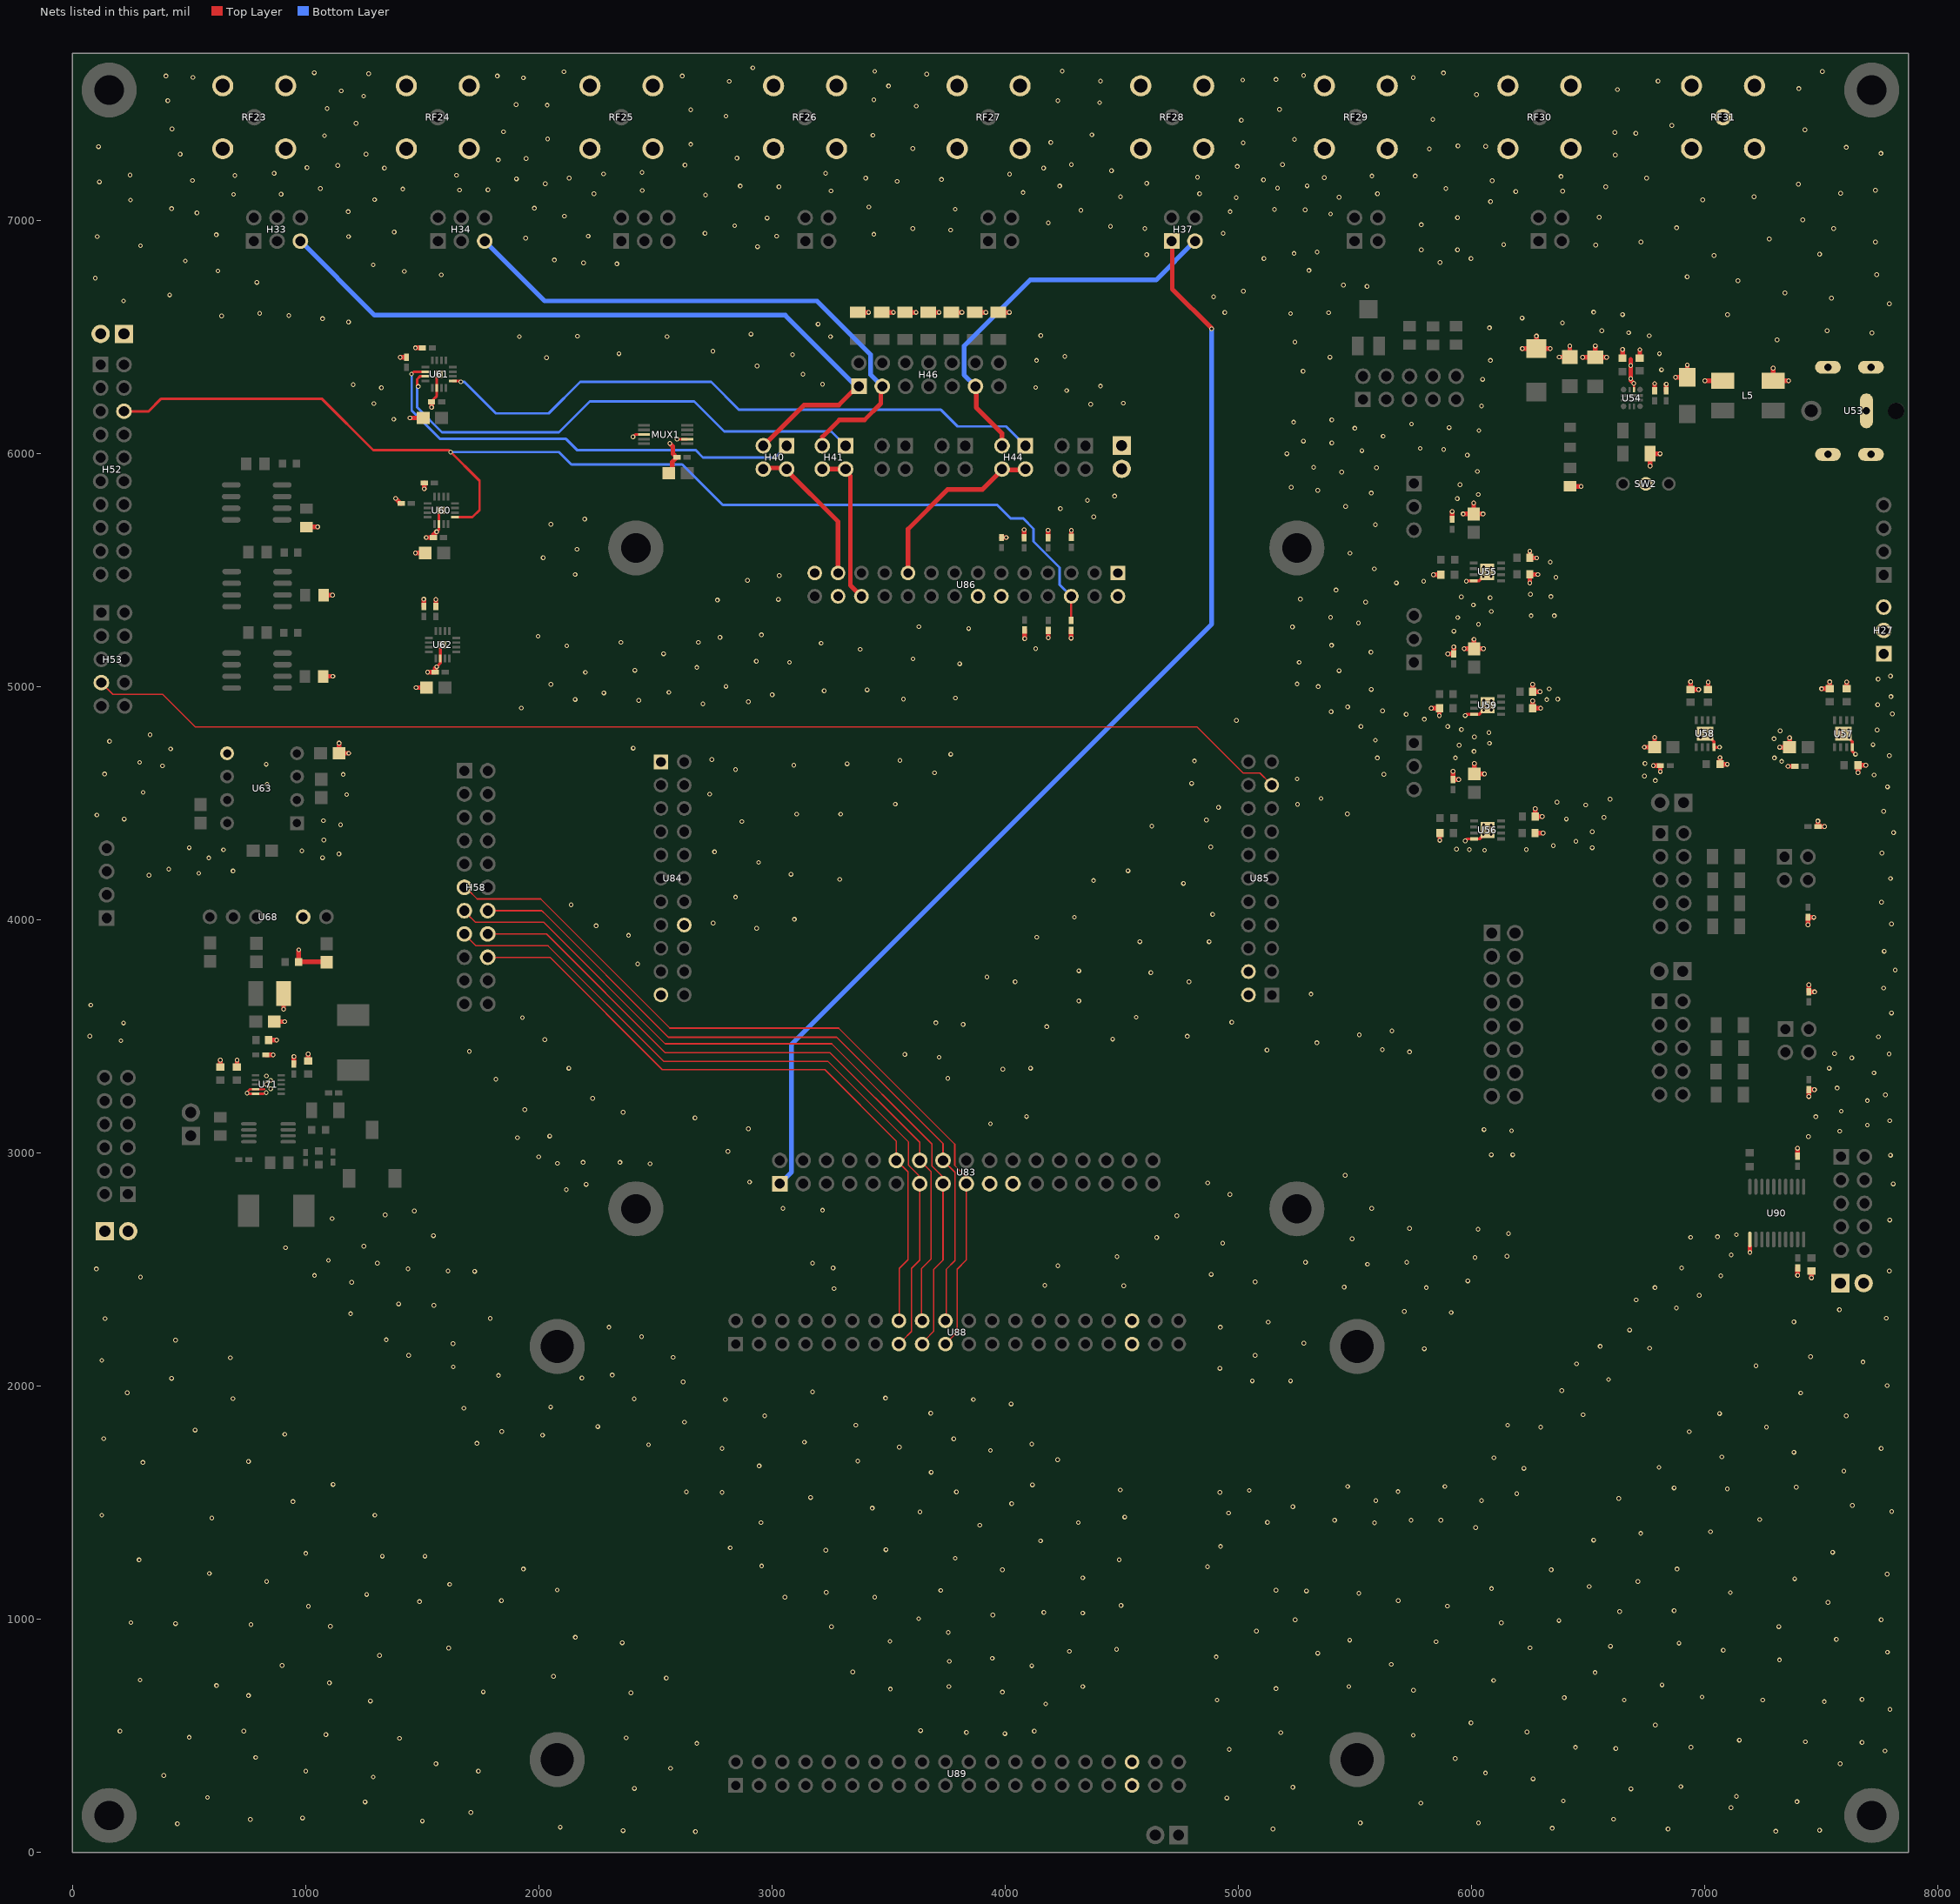
[diagram p0: the nets of this part, all layers, seen from the top]
# Altium PCB MISC62793.pcbdoc (part 5 of 6)
Units mil, origin at the board's own origin, x right, y up, seen from the top; angles counter-clockwise.
Board outline 7874.02 x 7716.54 mil, 4 copper layers (Top Layer, GND, VCC, Bottom Layer); 201 components, 197 nets, 941 pads, 1215 vias.

## Via types
v1: diameter 20, hole 12, Top Layer to Bottom Layer, 1215 vias

## Nets (pads, with @x,y where several pads share a name; then routed paths per layer and width w, separated by ;. In a path a pad name is that pad's centre, name@x,y a point inside that pad or via, vN(x,y) a via of type N, cw(c..) or ccw(c..) an arc to the next point about the centre after c; other vN are vias at no path point) (continued)
VSS: C126.1 C129.1 C130.1 C131.1 C132.1 C133.1 C134.1 C135.1 C136.1 C137.1 C138.1 C139.1 C140.1 C141.1 C142.1 C143.1 C144.1 C145.1 C146.1 C147.1 C148.1 C149.1 C150.1 C151.1 C152.1 C157.1 C158.1 C159.1 C163.1 C182.1 C183.1 C184.1 C185.2 C192.2 C193.2 C194.2 C195.1 C196.2 C197.1 C198.1 C199.1 C200.1 C201.1 C202.2 C203.2 C204.2 C205.2 C206.2 C207.2 C208.2 C215.1 C216.1 C217.1 C218.1 C219.1 C220.1 C221.1 C223.1 C224.1 C225.1 C226.1 C227.1 C228.1 D4.2 D5.1 H1.1 H1.2 H2.1 H2.2 H3.1 H3.2 H4.1 H4.2 H27.1 H27.2 H27.3 L5.2 L5.3 MUX1.3 MUX1.7 R91.1 R93.1 R96.1 R97.1 R98.1 R111.1 R113.1 R115.1 R120.2 R121.2 R122.2 R123.2 R124.2 R125.2 R126.2 R127.2 R134.2 R135.1 RF23.2 RF23.3 RF23.4 RF23.5 RF24.2 RF24.3 RF24.4 RF24.5 RF25.2 RF25.3 RF25.4 RF25.5 RF26.2 RF26.3 RF26.4 RF26.5 RF27.2 RF27.3 RF27.4 RF27.5 RF28.2 RF28.3 RF28.4 RF28.5 RF29.2 RF29.3 RF29.4 RF29.5 RF30.2 RF30.3 RF30.4 RF30.5 RF31.1 RF31.2 RF31.3 RF31.4 RF31.5 SW2.2 U53.2 U53.3 U54.8 U55.4 U55.9 U56.4 U56.9 U57.4 U57.9 U58.4 U58.9 U59.4 U59.9 U60.6 U60.17 U61.6 U61.17 U62.6 U62.17 U63.5 U68.2 U71.4 U71.5 U71.11 U82.2 U83.10 U83.11 U84.1 U84.16 U84.21 U85.2 U85.4 U86.1 U86.2 U86.12 U86.14 U86.26 U86.27 U88.35 U88.36 U89.35 U89.36 U90.11 | length 5722.7
  Top Layer w10: v1(749,3256) 749,3260 762.33,3273.33 U71.4@785.07,3273.33 821.67,3273.33 ; v1@750,3253.65 U71.5@785.07,3253.65 819.35,3253.65 ; v1(6696,6300.7) 6696.39,6300.31 U54.8@6696.39,6273.62
  Top Layer w11: C221.1@1544,6228 1562.85,6246.85 U61.6@1562.85,6281.39 U61.17@1562.85,6325.85 ; v1(1562,5664) 1572.28,5674.28 U60.6@1572.28,5697.2 U60.17@1572.28,5742.72 ; v1(2404,6071) 2414.06,6081.06 MUX1.3@2451.49,6081.06 ; v1(2593.37,6061.37) MUX1.7@2636.53,6061.37
  Top Layer w12: v1(1562.48,5085) 1577.9,5100.42 U62.6@1577.9,5119.95 U62.17@1577.9,5164.1
  Top Layer w13: v1(5973,4338) 5981.59,4346.59 U56.4@6010.83,4346.59 6034.59,4346.59 U56.9@6042,4354 ; v1(5973,4876) 5978.59,4881.59 U59.4@6010.83,4881.59 6033.59,4881.59 U59.9@6041,4889 ; v1(5978,5452) 5980.08,5454.08 U55.4@6009.98,5454.08 6033.08,5454.08 U55.9@6044,5465 ; U58.9@7033,4771 7040.3,4763.7 U58.4@7040.3,4740.08 v1(7063.92,4740.08) ; U57.9@7628,4769 7634.05,4762.95 U57.4@7634.05,4739.81 7634.05,4722.95 v1(7647,4710)
  Top Layer w20: C193.2@633.99,3367.61 v1(633.99,3397.99) ; C194.2@705.99,3367.61 v1(705.99,3397.99) ; C196.2@829.45,3420.05 v1(860.95,3420.05) ; C195.1@841.55,3484.05 v1(875.95,3484.05) ; C197.1@865.36,3563.05 v1(910.05,3563.05) ; v1(905.73,3616.27) C184.1@905.73,3683.05 ; C192.2@950,3381.46 v1(950,3413) ; v1(971,3871) 970.66,3870.66 R127.2@970.66,3819 C185.2@1078,3819 ; R111.1@1004.39,5684.7 v1(1051.7,5684.7) ; C183.1@1011,3393.56 v1(1011,3424) ; R115.1@1075.49,5044.07 v1(1116.93,5044.07) ; R113.1@1076.76,5392.07 v1(1115.93,5392.07) ; v1(1143.37,4757.37) C163.1@1143.37,4714 v1(1185,4714) ; v1(1386,5807) 1407.77,5785.23 C157.1@1410.86,5785.23 ; v1(1405.54,6412.46) C158.1@1433,6412.46 ; v1(1447.56,6152.44) C220.1@1504.32,6152.44 ; v1(1470.77,5573.23) C218.1@1512.95,5573.23 ; v1(1471,6453) C226.1@1500.54,6453 ; v1(1474,4996) C224.1@1518.63,4996 ; C159.1@1506.74,5343.47 v1(1506.74,5374.74) ; v1(1508.54,5848.46) C223.1@1508.54,5874 ; v1(1517.23,5639.23) C219.1@1548.86,5639.23 1548.86,5650.86 v1@1561,5663 ; v1(1523,5062.01) C225.1@1555.28,5062.01 1555.28,5077.28 v1@1562,5084 ; v1(1540.23,6198.23) C221.1@1540.23,6221.44 ; C227.1@1558.74,5343.47 v1(1558.74,5373.26) ; C228.1@2557.63,5915 2572,5929.37 2572,5963 C182.1@2591,5982 ; v1(2562,6043) 2575,6030 2575,5999 2591,5983 C182.1@2593.54,5983 ; R120.2@3368.53,6605.21 v1(3414.79,6605.21) ; R121.2@3470.53,6605.21 v1(3521.21,6605.21) ; R122.2@3570.53,6605.21 v1(3617.79,6605.21) ; R123.2@3669.53,6605.21 v1(3716.79,6605.21) ; R124.2@3769.53,6605.21 v1(3814.79,6605.21) ; R125.2@3870.53,6605.21 v1(3917.79,6605.21) ; R126.2@3970,6605.22 v1(4017.78,6605.22) ; C202.2@3985,5639.46 v1(4004.54,5639.46) ; C204.2@4082,5638.92 v1(4082,5673) ; v1(4084,5206) C203.2@4084,5242.54 ; C206.2@4184,5637.92 v1(4184,5671) ; v1(4185,5209) C205.2@4185,5240.54 ; v1(4283,5208) C207.2@4283,5240.54 ; C208.2@4284,5639.92 v1(4284,5670) ; v1(5828.01,4906.99) R93.1@5862.27,4906.99 v1(5862.27,4875.27) ; v1(5837.33,5479.67) R91.1@5868.13,5479.67 ; v1(5864.27,4340.73) R96.1@5864.27,4371.99 ; v1(5898.46,5140.46) C145.1@5924,5140.46 v1(5924,5170) ; C144.1@5917,5717.46 v1(5917,5751) ; v1(5921,4637) C146.1@5921,4601.46 v1(5945.46,4601.46) ; v1(5964.36,5740.36) C131.1@6009.51,5740.36 ; v1(5968.36,5162.36) C134.1@6010.93,5162.36 ; v1(6009.51,5787.51) C131.1@6009.51,5740.36 ; v1(6010.93,5202.93) C134.1@6010.93,5162.36 ; v1(6011.93,4669.93) C137.1@6011.93,4625.36 v1(6055.64,4625.36) ; v1(6049.64,5740.36) C131.1@6009.51,5740.36 ; v1(6051.64,5162.36) C134.1@6010.93,5162.36 ; v1(6217.93,6449.93) D4.2@6278.53,6449.93 ; v1(6250.25,5444.75) C130.1@6250.25,5480.98 v1(6284.98,5480.98) ; v1(6250.25,5581.25) C129.1@6250.25,5551.85 v1(6279.85,5551.85) ; v1(6262.49,4938.51) C133.1@6262.49,4906.99 v1(6297.01,4906.99) ; v1(6262.49,5009.49) C132.1@6262.49,4977.99 v1(6293.99,4977.99) ; C136.1@6272.49,4371.99 v1(6306.99,4371.99) ; v1(6273.49,4476.49) C135.1@6273.49,4442.99 v1(6302.99,4442.99) ; v1(6278.53,6503.53) D4.2@6278.53,6449.93 ; v1(6338.07,6449.93) D4.2@6278.53,6449.93 ; v1(6376.3,6413.7) C201.1@6422,6413.7 v1(6422,6461) ; R135.1@6422,5858.63 v1(6470.37,5858.63) ; v1(6476.69,6412.69) C200.1@6530.53,6412.69 ; v1(6530.53,6461.53) C200.1@6530.53,6412.69 ; v1(6579.69,6412.69) C200.1@6530.53,6412.69 ; R134.2@6648,6409.66 v1(6648,6446) ; 6683,6404 v1(6683,6377) 6683,6362 v1(6683,6321) 6683,6313.7 v1(6696,6300.7) ; C126.1@6722,6409.56 v1(6722,6445) ; v1(6741.18,4740.18) C142.1@6785.53,4740.18 v1(6785.53,4782.53) ; v1(6765.75,5946.25) U82.2@6765.75,5998.99 v1(6809.01,5998.99) ; v1(6780,4661) C148.1@6809.54,4661 v1(6809.54,4635.46) ; C198.1@6785.53,6269.45 v1(6785.53,6299.53) ; C199.1@6835.53,6269.45 v1(6835.53,6297.53) ; v1(6875.27,6326.73) D5.1@6925.53,6326.73 v1(6925.53,6379.53) ; v1(6939.9,5020.9) C141.1@6939.9,4987.74 v1(6974.26,4987.74) ; v1(7001.03,6311.97) L5.3@7077.26,6311.97 ; C143.1@7014.9,4987.74 v1(7014.9,5019.1) ; v1(7065.66,4695.66) R98.1@7065.66,4667 v1(7097,4667) ; v1(7193.98,2573.02) U90.11@7193.98,2596 ; v1(7293.8,6365.8) L5.2@7293.8,6311.97 v1(7359.97,6311.97) ; v1(7321.91,4739.91) C139.1@7364.28,4739.91 v1(7364.28,4780.28) ; v1(7357,4658) C147.1@7387.54,4658 ; C215.1@7398,2985.46 v1(7398,3020) ; v1(7399,2475) C217.1@7399,2506.54 ; v1(7443,3978) C152.1@7443,4010.54 v1(7468.54,4010.54) ; v1(7447,3242) C150.1@7447,3271.54 v1(7470.54,3271.54) ; v1(7447,3721) C149.1@7447,3690.46 v1(7471.54,3690.46) ; v1(7458,2464) C216.1@7458,2493.44 ; v1(7485.46,4423.46) C151.1@7485.46,4400 v1(7514,4400) ; v1(7501.47,4990.47) C138.1@7536.65,4990.47 v1(7536.65,5020.35) ; C140.1@7609,4990.56 v1(7609,5020) ; v1(7657.66,4631.34) R97.1@7657.66,4663 v1(7691,4663)
  Bottom Layer w10: v1@6696,6298 v1(6696,6300.7)
  other v1: 2672,89 7305,90 2362,93 7493,94 5149,100 6843,100 6346,103 2092,108 450,122 5523,126 6030,126 1501,134 763,141 6609,142 987,147 1709,171 7113,191 5783,211 1255,216 7396,217 6394,220 4951,233 579,235 7136,240 6684,272 2410,274 5234,279 6898,282 6264,315 1290,323 392,329 6060,340 1001,348 1741,348 2565,360 1559,380 7581,380 5930,402 786,407 7773,435 4961,441 6619,445 6446,450 6941,451 2678,467 7675,471 7432,474 7149,481 1403,489 2375,491 501,493 5750,502 1087,505 3999,509 5182,513 3834,514 6238,516 204,520 735,520 4125,520 3638,522 6788,546 5998,555 7795,613 4174,636 7513,646 1278,649 4909,653 6655,653 7249,653 7675,656 6398,663 6989,666 755,672 2395,684 3988,687 1762,688 5751,695 3508,700 5162,702 3759,711 4333,711 5474,711 618,715 6817,718 1102,727 6095,737 290,739 2547,747 2063,755 6530,771 3347,773 4114,800 899,801 5656,806 3761,819 7321,825 3945,832 4905,838 1317,844 5341,854 7784,858 4276,862 7080,867 4478,870 1614,876 6251,877 6596,884 6890,897 2358,899 5848,903 3506,905 5478,910 7565,913 2157,922 3756,943 5078,949 3255,967 7318,968 1106,969 766,977 442,981 6128,984 251,985 6375,994 5244,997 7757,997 3629,1002 3947,1018 4333,1026 4166,1029 6635,1033 6869,1036 1012,1055 5897,1056 4497,1059 7529,1072 1489,1075 1840,1079 5686,1079 3056,1094 3441,1094 1262,1106 5517,1111 7110,1114 3233,1115 5292,1121 3724,1123 5162,1124 2079,1125 6086,1131 6505,1140 1618,1149 833,1161 6714,1161 7386,1173 4333,1177 7783,1193 587,1196 3988,1212 6342,1212 1934,1215 6882,1215 4868,1225 2956,1228 286,1254 4489,1255 3786,1261 1329,1270 1512,1270 1001,1282 7549,1287 3231,1296 3489,1298 2821,1306 4924,1312 4152,1336 6524,1339 6726,1368 7025,1375 6018,1393 3891,1403 5584,1413 2953,1414 4314,1414 5125,1415 5413,1424 5741,1424 5869,1424 7236,1427 598,1434 4513,1438 126,1446 1297,1446 4958,1455 3635,1460 7802,1462 3430,1476 5234,1482 7633,1488 4028,1495 946,1504 5590,1508 6043,1508 6632,1518 3166,1522 6194,1538 2786,1544 4921,1544 2633,1546 3791,1546 5685,1547 5047,1552 4494,1554 7097,1559 6869,1563 7393,1566 5469,1569 5886,1569 4117,1576 1118,1578 3683,1630 7597,1635 6225,1647 6804,1651 2945,1657 302,1672 755,1676 3368,1678 4225,1684 6096,1692 7074,1696 7383,1716 3937,1724 2786,1732 7757,1732 3546,1738 2471,1748 4114,1751 1735,1754 3139,1759 3780,1773 134,1774 2016,1789 911,1793 6934,1804 1841,1805 526,1811 6297,1824 7265,1824 2253,1826 3360,1832 6155,1832 2625,1845 2969,1872 7607,1872 6479,1877 7064,1882 3681,1883 1679,1905 2051,1910 4026,1923 2800,1942 3864,1942 2409,1945 688,1946 3487,1948 7412,1970 235,1971 3174,1975 6387,1980 7783,2002 2619,2018 5060,2022 5224,2022 6588,2028 425,2033 2185,2034 1827,2045 2315,2047 4921,2076 1633,2082 7220,2087 6451,2095 7679,2103 126,2110 677,2121 2576,2123 7454,2126 1442,2131 5072,2131 5798,2160 6764,2162 6552,2170 1632,2182 5281,2184 442,2197 1346,2198 2441,2212 6678,2240 2301,2252 4923,2252 5128,2274 7383,2275 140,2289 1792,2290 7779,2291 1193,2310 5913,2315 5712,2320 7578,2327 6879,2335 1550,2346 1399,2352 6706,2369 6977,2389 3266,2418 5806,2422 6787,2422 5454,2424 4509,2430 4170,2432 1198,2445 5072,2447 5984,2451 292,2467 7069,2473 1038,2474 4884,2479 1725,2492 1611,2493 7792,2493 103,2502 1439,2503 3262,2506 6901,2506 4226,2516 5554,2522 1308,2527 3174,2527 5288,2531 5722,2531 1098,2539 6015,2551 4480,2555 6152,2557 7114,2562 914,2593 1250,2600 4933,2613 5488,2631 4650,2637 6940,2638 7055,2640 1548,2645 7136,2649 6159,2654 6028,2672 5734,2676 7794,2712 1114,2718 4736,2730 1341,2734 1466,2751 3217,2754 3047,2762 5572,2762 4964,2822 2118,2842 2203,2865 7809,2867 4869,2871 2904,2875 5458,2904 2477,2953 2080,2955 2190,2959 2348,2959 2000,2983 7797,2990 6085,2992 6177,2992 2811,3006 1908,3065 7445,3070 2047,3072 7579,3093 6172,3095 6054,3100 2899,3103 7698,3119 3937,3125 7794,3138 2670,3150 7477,3155 4092,3156 2362,3174 7586,3179 1940,3185 7698,3224 2231,3234 7775,3249 831,3258 850,3275 7568,3278 832,3294 850,3311 1816,3316 3754,3320 832,3330 7726,3343 3990,3359 2129,3363 4109,3363 7534,3363 7631,3407 3717,3410 3570,3422 7791,3424 7557,3426 5734,3433 1702,3435 5123,3441 5618,3443 5337,3472 208,3481 2026,3486 4461,3488 7745,3498 4781,3500 75,3501 5519,3506 5659,3523 4179,3541 3820,3551 219,3557 3703,3558 4972,3560 1930,3580 4562,3582 7801,3600 79,3634 4316,3652 5312,3681 7768,3707 4043,3734 4789,3734 3922,3754 4625,3773 4316,3781 7817,3784 2424,3810 7770,3865 4578,3906 4875,3906 4136,3925 2385,3933 2934,3963 2246,3974 7801,3982 2748,3986 3096,4002 4297,4011 4890,4023 2139,4064 7758,4075 2844,4097 4765,4156 4379,4168 3291,4173 7797,4177 328,4191 3082,4195 542,4199 689,4209 4527,4210 413,4217 2943,4246 585,4265 1073,4266 1143,4282 7760,4286 2754,4291 984,4295 6056,4298 648,4300 5991,4301 6235,4301 5936,4303 501,4309 6518,4309 4882,4312 6351,4318 6448,4336 1078,4342 6051,4365 6084,4366 7810,4374 6518,4377 6067,4386 4629,4402 6084,4405 1150,4407 6052,4408 2871,4421 1076,4425 4863,4428 222,4432 6407,4432 6568,4439 105,4449 3106,4453 3295,4453 5468,4454 7768,4465 4915,4482 6490,4492 5254,4495 3529,4496 6367,4504 6594,4517 5355,4520 1176,4537 2733,4539 303,4546 7784,4570 835,4581 4800,4585 6788,4597 5252,4604 6742,4616 7727,4621 1161,4623 5624,4624 138,4625 3697,4630 2844,4644 386,4660 3094,4663 831,4667 3322,4669 6744,4670 288,4675 7330,4679 4812,4681 3549,4683 2742,4687 5596,4694 5931,4694 7299,4694 7792,4704 3767,4710 6011,4722 421,4733 2405,4736 5947,4749 7722,4751 6077,4757 159,4765 5588,4770 7298,4776 7025,4781 6982,4782 7619,4782 7576,4783 6012,4784 333,4793 7004,4797 7598,4798 6075,4803 7324,4810 6985,4814 7024,4814 7740,4814 7579,4815 7618,4815 5957,4816 5526,4829 5898,4829 4992,4855 5798,4860 5720,4881 7805,4883 5398,4892 5619,4896 6052,4899 6085,4900 1925,4908 5469,4913 6068,4920 7742,4922 2704,4926 2899,4935 6085,4939 2429,4941 6053,4942 6323,4944 2156,4945 3564,4946 6370,4946 3787,4951 7799,4957 3001,4965 2279,4973 2558,4975 3224,4982 3408,4986 5570,4988 6333,4990 5343,5000 2803,5001 2052,5010 5252,5011 7744,5032 7797,5045 2200,5061 5432,5068 2412,5070 2678,5082 3805,5098 3075,5104 5261,5104 2933,5109 3605,5119 2535,5141 5569,5148 3378,5160 4131,5163 2120,5175 5400,5177 1588,5179 3211,5186 2352,5190 2684,5190 2777,5211 1997,5216 2955,5222 5925,5238 3844,5249 5232,5256 3630,5257 6030,5267 5515,5273 5941,5296 5396,5297 6256,5304 6355,5304 6085,5322 6008,5350 5546,5362 2766,5371 3028,5374 5266,5375 6080,5381 5956,5385 6341,5386 6253,5396 5419,5414 5678,5445 5795,5452 2895,5456 6362,5469 6051,5471 6084,5472 3031,5476 2156,5481 6067,5492 5583,5505 6084,5511 6052,5514 6338,5534 2019,5553 5479,5572 2164,5589 5588,5694 2052,5696 2197,5719 4380,5728 1582,5756 4237,5763 5460,5773 4353,5799 5939,5806 4470,5817 6029,5824 5570,5830 5341,5842 5227,5855 5951,5866 5443,5920 6025,5923 5593,5939 5323,5941 5982,5993 5208,5999 5530,6012 5881,6017 5780,6022 5401,6045 5279,6053 5621,6074 6032,6098 5500,6108 5904,6111 5743,6126 5237,6134 5401,6144 1378,6147 6043,6204 4367,6211 1293,6214 4507,6216 4264,6270 1325,6282 4131,6283 4409,6289 1204,6295 3217,6297 6048,6318 3133,6340 1572,6341 5278,6353 6815,6359 2936,6375 4135,6399 6081,6399 2033,6411 5393,6413 4256,6416 3088,6424 2344,6428 6806,6428 2747,6439 5243,6478 7311,6487 1917,6501 2550,6501 3251,6501 2166,6503 6762,6505 4153,6506 2910,6512 7717,6517 6674,6518 6559,6526 7525,6526 6077,6539 3198,6555 6390,6560 1184,6564 1073,6578 6217,6581 640,6590 928,6592 7098,6595 6648,6596 5224,6600 803,6601 5387,6604 4942,6605 6524,6606 7792,6642 219,6654 7544,6666 4894,6672 417,6680 7344,6689 5022,6696 5552,6717 5451,6722 791,6734 7143,6741 98,6752 6925,6758 1582,6766 7738,6767 1423,6781 624,6783 5303,6785 1290,6809 2335,6813 2192,6817 5865,6819 484,6826 2067,6830 5110,6836 5998,6836 7040,6849 4607,6853 7493,6855 5239,6858 5338,6864 5785,6873 5940,6873 2938,6887 292,6891 6533,6894 6138,6896 6727,6907 7732,6907 7277,6920 1944,6924 106,6930 1184,6930 2212,6932 3020,6932 617,6938 3437,6940 2713,6944 4935,6944 1380,6950 3766,6958 3604,6965 4599,6965 7553,6965 6880,6968 4452,6974 2840,6977 5785,6981 4185,6989 7421,7002 2979,7010 5940,7011 6548,7013 2110,7018 5396,7027 534,7032 1183,7037 4965,7037 4325,7043 5287,7045 5155,7047 3786,7048 425,7050 1981,7052 3416,7057 6082,7080 249,7087 6992,7088 1296,7089 4991,7097 5432,7099 4495,7101 7212,7101 2715,7108 691,7111 895,7112 2237,7114 4834,7114 5597,7114 7583,7116 4077,7119 6190,7123 6391,7125 3253,7126 2444,7128 7732,7129 1660,7130 1782,7131 1417,7134 1063,7136 5890,7136 5168,7138 3030,7144 6576,7144 2864,7147 4234,7147 5295,7148 7402,7155 2028,7157 4607,7159 116,7165 3537,7167 6089,7170 515,7171 5108,7174 3727,7175 1904,7178 2130,7181 3402,7181 6751,7181 5369,7183 4825,7185 6384,7188 5573,7190 5759,7190 697,7192 1647,7193 247,7194 4019,7198 2278,7199 865,7202 3230,7202 2443,7205 4456,7213 1338,7224 4165,7224 1006,7226 4996,7231 1138,7235 2627,7237 4284,7239 5190,7239 1826,7259 1946,7265 2850,7267 6617,7280 462,7284 1259,7284 7756,7287 5819,7306 3604,7308 7607,7313 112,7316 6061,7317 5942,7319 2652,7326 5021,7332 4196,7334 5241,7347 2038,7349 1081,7363 3433,7365 4372,7367 6705,7373 6615,7377 1849,7380 7430,7388 427,7392 6859,7407 1216,7416 5013,7429 5834,7433 2803,7447 2652,7474 5177,7476 1092,7480 3619,7490 2036,7494 1903,7496 4405,7505 409,7513 4226,7513 3437,7517 1249,7533 6022,7539 1153,7555 6626,7561 7404,7565 3500,7576 2817,7596 4409,7597 6800,7597 5019,7602 5162,7604 1934,7611 5750,7612 517,7613 401,7619 1822,7619 2615,7619 5280,7621 3664,7627 1270,7629 5880,7632 1037,7633 2108,7637 7505,7638 3441,7639 4245,7640 2918,7654
VTH_CMP: C207.1 H52.6 U60.9 U86.6 | length 4995
  Top Layer w11: H52.6@236,6181 327,6181 381,6235 1069,6235 1290,6014 1615,6014 1746,5883 1746,5757 1715.72,5726.72 U60.9@1641.18,5726.72 ; C207.1@4283,5283.46 U86.6@4283,5364
  Bottom Layer w11: v1(1622,6006) 2087,6006 2140,5953 2615,5953 2789,5779 3966,5779 4023,5722 4077,5722 4122,5677 4122,5623 4234,5511 4234,5436.96 U86.6@4283.65,5387.31
VWL1: H40.2 H40.4 U86.25 | length 647.2
  Top Layer w20: H40.4@2952,5938 3053,5938 3283.65,5707.35 U86.25@3283.65,5487.31
VWL1_BNC: H33.5 H40.3 H46.1 | length 3141.7
  Top Layer w20: H40.3@2963,6033 3138,6208 3287,6208 H46.1@3354,6275
  Bottom Layer w20: H33.5@977.64,6911 1295.64,6593 2578,6593 ; 2553,6593 2578,6593 ; H46.1@3350,6300 3057,6593 2578,6593
VWL1_DAC: H40.1 U61.2 | length 1910.9
  Top Layer w11: v1@1457,6344 1463.28,6350.28 U61.2@1513.64,6350.28
  Bottom Layer w11: v1(1454,6341) v1@1455.5,6339.5 ; v1@1455,6339 1455,6184 1577,6062 2117,6062 2164,6015 2672,6015 2704,5983 3014,5983 H40.1@3051,6020
VWL2: H41.2 H41.4 U86.24 | length 659.9
  Top Layer w20: H41.4@3224,5933 3306,5933 3336.16,5902.84 3336.16,5434.8 U86.24@3383.65,5387.31
VWL2_BNC: H34.5 H41.3 H46.3 | length 2430.7
  Top Layer w20: H41.3@3216,6033 3216,6071 3289,6144 3397,6144 3467,6214 H46.3@3467,6283
  Bottom Layer w20: H34.5@1768,6911 2025,6654 3193,6654 3422.46,6424.54 3422.46,6338.54 H46.3@3473,6288
VWL2_DAC: H41.1 U61.3 | length 2174.2
  Top Layer w11: v1@1478,6292 1478,6318 1490.6,6330.6 U61.3@1513.64,6330.6
  Bottom Layer w11: v1@1484,6288 v1(1483,6287) 1479,6283 1479,6197 1585,6091 2087,6091 2219,6223 2667,6223 2795,6095 3254,6095 H41.1@3316,6033
VWL_DARK: H44.2 H44.4 U86.19 | length 784.6
  Top Layer w20: U86.19@3583.65,5487.31 3583.65,5675.65 3753,5845 3902,5845 3986,5929 H44.2@4075,5929
VWL_DARK_BNC: H37.3 H44.3 H46.11 | length 1684.3
  Top Layer w20: H46.11@3876,6301 3876,6197 3987,6086 H44.3@3987,6033
  Bottom Layer w20: H46.11@3873,6288 3823.54,6337.46 3823.54,6460.54 4107,6744 4647.21,6744 H37.3@4814.21,6911
VWL_DARK_DAC: H44.1 U61.9 | length 2680.2
  Top Layer w11: U61.9@1631.75,6310.91 1662.09,6310.91 v1(1666,6307)
  Bottom Layer w11: v1@1668,6307 1681,6307 1816,6172 2043,6172 2178,6307 2739,6307 2859,6187 3725,6187 3796,6116 4004,6116 H44.1@4087,6033
WE_CTRL: H58.11 U83.9 U88.19 | length 3434.2
  Top Layer w6: H58.11@1696,4129 1736,4089 2008,4089 2562,3535 3286,3535 3784,3037 3784,2946 3833.65,2896.35 U83.9@3833.65,2867.63 3833.65,2540.65 3794,2501 3794,2231 U88.19@3758,2195
WELL: H37.1 U83.1 | length 4882.6
  Top Layer w20: H37.1@4717,6914 4717,6911 4717,6705 v1@4886,6536
  Bottom Layer w20: U83.1@3033.66,2867.62 3084,2917.95 3084,3466 4886,5268 v1(4886,6535)
WL_ADDR0: H58.18 U83.29 U88.16 | length 2879.4
  Top Layer w6: H58.18@1781,3839 2048,3839 2530,3357 3227,3357 3533.65,3050.35 U83.29@3533.65,2967.63 3583,2918.28 3583,2542 3546,2505 3546,2335 ; U88.16@3546,2297 3546,2335 ; 3546,2324 3546,2335
WL_ADDR1: H58.15 U83.7 U88.15 | length 3157.8
  Top Layer w6: H58.15@1693,3926 1731,3888 2040,3888 2535,3393 3239,3393 3586,3046 3586,2947 3633.65,2899.35 U83.7@3633.65,2867.63 3633.65,2539.65 3598,2504 3598,2234 U88.15@3560,2196
WL_CTRL: H58.14 U83.27 U88.20 | length 3150.7
  Top Layer w6: H58.14@1781,4039 2013,4039 2018,4034 2021,4031 2556,3496 3278,3496 3733.65,3040.35 U83.27@3733.65,2967.63 3785,2916.28 3785,2538 3747,2500 3747,2336 ; U88.20@3747,2298 3747,2336 ; 3747,2331 3747,2336
WL_D_ADDR0: H58.16 U83.28 U88.18 | length 3026.6
  Top Layer w6: H58.16@1781,3939 2033,3939 2542,3430 3249,3430 3633.65,3045.35 U83.28@3633.65,2967.63 3683,2918.28 3683,2546 3642,2505 3642,2333 ; U88.18@3642,2288 3642,2333 ; 3642,2324 3642,2333
WL_D_ADDR1: H58.13 U83.8 U88.17 | length 3297.1
  Top Layer w6: H58.13@1690,4027 1727,3990 2020,3990 2542,3468 3256,3468 3686,3038 3686,2944 3733.65,2896.35 U83.8@3733.65,2867.63 3733.65,2539.65 3694,2500 3694,2235 U88.17@3657,2198
WL_TEST: H53.7 U85.19 | length 5198.6
  Top Layer w6: H53.7@126,5014 173,4967 387,4967 527,4827 4823,4827 5021,4629 5093,4629 U85.19@5135,4587 ; U85.19@5134.48,4586.48 U85.19@5143.5,4577.46
pads on no net: H53.2 H60.2 R119.3 SW2.1 U53.0 U54.2 U54.3 U54.4 U54.10 U60.15 U61.15 U62.15 U64.1 U64.5 U64.8 U65.1 U65.5 U65.8 U66.1 U66.5 U66.8 U83.18 U84.22 U85.17 U85.22 U86.23 U89.9 U89.11 U89.13 U89.15 U89.17 U89.18 U89.19 U89.20 U89.21 U89.22 U89.23 U89.24 U89.25 U89.26 U89.27 U89.29 U89.31 U89.33 U90.6 U90.7 U90.8 U90.9 U90.12 U90.13 U90.14 U90.15

## Polygon pours and split planes (outlines as drawn)
AVDD on Top Layer "Bottom Layer-No Net" (solid, remove dead copper, pour order 1010): 3911,5085 3911,5068 3911,4966 3917,4960 3924,4953 3938,4953 5051,4953 5051,4951 5882,4120 5888,4114 5971,4114 6250,4114 6420,3944 6440,3924 6499,3924 6819,3924 6841,3946 6848,3953 6848,3968 6848,4528 6835,4541 6832,4544 6817,4544 6705,4544 6682,4521 6666,4505 6666,4444 6666,4372 6597,4303 6545,4251 6438,4251 5922,4251 5775,4398 5073,5100 3927,5100 3920,5100 3912,5092 3911,5091 3911,5085
1P8V on Top Layer "Bottom Layer-No Net" (solid, remove dead copper, pour order 1009): 5675,4768 5675,4553 5717,4511 5730,4498 5769,4498 5797,4498 5805,4490 5822,4473 5822,4453 5822,4433 5827,4428 5838,4417 5850,4417 5873,4417 5877,4421 5879,4423 5879,4428 5879,4461 5889,4471 5891,4473 5917,4473 5950,4473 5957,4466 5962,4461 5962,4449 5962,4401 5965,4398 5972,4391 5990,4391 6021,4391 6023,4393 6027,4397 6027,4410 6027,4470 6041,4484 6049,4492 6049,4507 6049,4564 6042,4571 6039,4574 5997,4574 5897,4574 5888,4583 5866,4605 5866,4650 5866,4769 5835,4800 5826,4809 5803,4809 5694,4809 5683,4798 5675,4790 5675,4769
DAC_VDD on Top Layer "Bottom Layer-No Net" (solid, remove dead copper, pour order 1008): 5693,5857 5693,5562 5714,5541 5730,5525 5854,5525 5880,5525 5882,5527 5884,5529 5884,5534 5884,5572 5891,5579 5894,5582 5909,5582 5962,5582 5964,5580 5970,5574 5970,5561 5970,5509 5976,5503 5982,5497 5995,5497 6022,5497 6025,5500 6027,5502 6027,5510 6027,5587 6038,5598 6049,5609 6049,5618 6049,5674 6036,5687 6033,5690 5997,5690 5883,5690 5876,5697 5869,5704 5869,5721 5869,5906 5853,5922 5852,5923 5828,5923 5718,5923 5710,5915 5693,5898 5693,5857
3P3V on Top Layer "Bottom Layer-No Net" (solid, remove dead copper, pour order 1007): 5665,5282 5665,4972 5677,4960 5688,4949 5829,4949 5871,4949 5875,4953 5877,4955 5877,4964 5877,4995 5883,5001 5885,5003 5896,5003 5947,5003 5950,5000 5959,4991 5959,4978 5959,4934 5962,4931 5967,4926 5988,4926 6022,4926 6025,4929 6026,4930 6026,4938 6026,5009 6037,5020 6043,5026 6043,5051 6043,5101 6037,5107 6031,5113 5983,5113 5890,5113 5875,5128 5857,5146 5857,5179 5857,5341 5833,5365 5830,5368 5810,5368 5700,5368 5687,5355 5665,5333 5665,5282
LDO_DVDD on Top Layer "Bottom Layer-No Net" (solid, remove dead copper, pour order 1006): 7416,4713 7416,4608 7477,4547 7545,4479 7545,4291 7545,3692 7524,3671 7517,3664 7450,3664 7436,3664 7430,3658 7414,3642 7414,3540 7414,3520 7428,3506 7438,3496 7460,3496 7597,3496 7653,3552 7690,3589 7690,3905 7690,4519 7638,4571 7614,4595 7614,4718 7614,4746 7609,4751 7604,4756 7590,4756 7505,4756 7495,4766 7491,4770 7474,4770 7426,4770 7419,4763 7416,4760 7416,4713